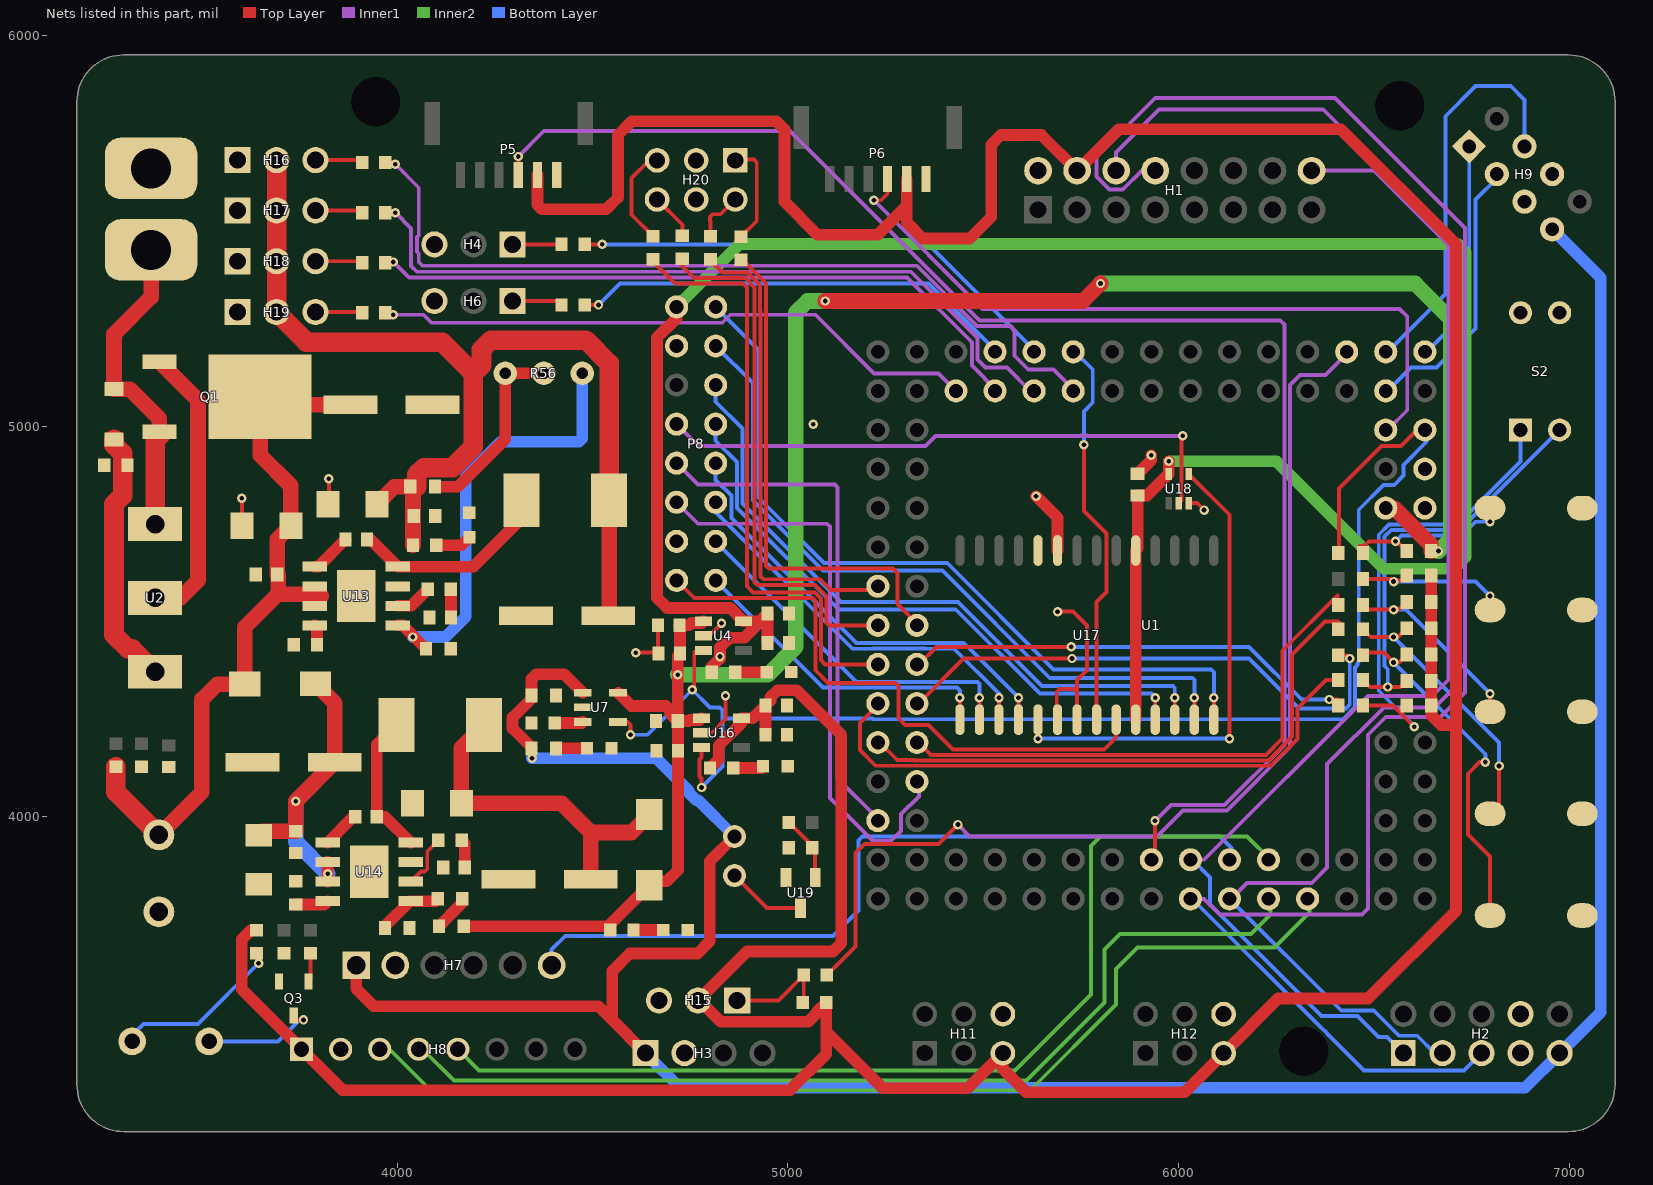
[diagram p0: the nets of this part, all layers, seen from the top]
# Altium PCB MISC49918.pcbdoc (part 2 of 2)
Units mil, origin at the board's own origin, x right, y up, seen from the top; angles counter-clockwise.
Board outline 3937.01 x 2755.91 mil, 4 copper layers (Top Layer, Inner1, Inner2, Bottom Layer), stack 62.447 mil thick; 130 components, 134 nets, 493 pads, 82 vias.

## Via types
v1: diameter 24.02, hole 12, Top Layer to Bottom Layer, 82 vias

## Nets (pads, with @x,y where several pads share a name; then routed paths per layer and width w, separated by ;. In a path a pad name is that pad's centre, name@x,y a point inside that pad or via, vN(x,y) a via of type N, cw(c..) or ccw(c..) an arc to the next point about the centre after c; other vN are vias at no path point) (continued)
7.3: U1.25 U17.8 | length 1003.8
  Top Layer w10: v1(5757.5,4952.5) 5757.5,4782.5 5815,4725 5815,4575 5790,4550 U17.8@5790,4248.46
  Bottom Layer w10: U1.25@5734.65,5190 5780,5144.65 5780,5060 5757.5,5037.5 v1(5757.5,4952.5)
7.4: R83.1 U1.45 | length 1218.1
  Top Layer w10: R83.1@4805,5420.34 4832.48,5392.86 4896.78,5392.86 4928.84,5360.81 4928.84,5294.02 4930,5292.86 4930,4615 4937.07,4607.93 5082.07,4607.93 5110,4580 5224.65,4580 U1.45@5234.65,4590
7.5: R61.2 U1.47 | length 1378.5
  Top Layer w10: R61.2@4730,5420.34 4730,5408.85 4760,5378.85 4890.98,5378.85 4914.82,5355 4914.82,4600 4921.89,4592.93 5069.64,4592.93 5098.03,4564.54 5098.03,4497.07 5105.1,4490 U1.47@5234.65,4490
7.6: R63.1 U1.48 | length 1312
  Top Layer w10: R63.1@4880,5425.34 4884.12,5425.34 4944.02,5365.45 4944.02,4642.07 4951.09,4635 5268.44,4635 5280,4623.44 5280,4544.65 U1.48@5334.65,4490
7.7: R62.2 U1.49 | length 1546.3
  Top Layer w10: R62.2@4655.62,5420.34 4711.13,5364.83 4885.17,5364.83 4895,5355 4895,4590 4910.98,4574.02 5068.73,4574.02 5084.02,4558.73 5084.02,4400.98 5095,4390 U1.49@5234.65,4390
8.0: P5.3 U1.74 | length 3829.6
  Top Layer w10: P5.3@4309.61,5642.32 4310,5642.72 v1(4310,5690) ; U1.74@5934.65,3890 5939.46,3894.81 v1(5939.46,3989.46)
  Inner1 w10: v1(4310,5690) 4375,5755 5005,5755 5490,5270 6260,5270 6270.51,5259.49 6270.51,4183.16 6117.35,4030 5980,4030 v1(5939.46,3989.46)
8.1: H1.8 H2.5 U1.75 | length 4720.8
  Inner1 w10: H1.8@5940,5653.7 5905.64,5653.7 5856.94,5605 5823.06,5605 5789.15,5638.91 5789.15,5689.15 5940,5840 6400,5840 6733.06,5506.94 6733.06,4318.06 6670,4255 6530,4255 6485,4210 6485,3765 6469.49,3749.49 6105.51,3749.49 6065,3790 U1.75@6034.65,3790
  Bottom Layer w10: U1.75@6034.65,3790 6363.9,3460.74 cw(c6320.01,3400.01) 6380.74,3443.9 6474.09,3350.55 6730.55,3350.55 H2.5@6775,3395
8.2: H1.16 H2.1 U1.76 | length 3174.3
  Inner1 w10: U1.76@6034.65,3890 6065,3890 6484.02,4309.02 6649.02,4309.02 6690,4350 6690,5463.7 6500,5653.7 H1.16@6340,5653.7
  Bottom Layer w10: U1.76@6035,3890 6080,3845 6080,3775 6365,3490 6457.53,3490 6511,3436.54 6533.46,3436.54 H2.1@6575,3395
8.3: H1.6 H2.3 U1.77 | length 3902.6
  Inner1 w10: H1.6@5840,5653.7 5840,5700 5950,5810 6370,5810 6710,5470 6710,4335 6655,4280 6525,4280 6380,4135 6380,3870 6340.51,3830.51 6175.16,3830.51 U1.77@6134.65,3790
  Bottom Layer w10: U1.77@6130,3790 6415.98,3504.02 6499.2,3504.02 6563.76,3439.45 6610.55,3439.45 6655,3395 H2.3@6675,3395
8.4: H7.6 U1.78 | length 2047.4
  Bottom Layer w10: H7.6@4395,3620 4395,3660 4430,3695 5115.18,3695 5180,3759.82 5180,3939.49 5190,3949.49 6105.51,3949.49 6135,3920 U1.78@6135,3890
8.5: H8.4 U1.79 | length 2508.3
  Inner2 w10: H8.4@4055.01,3405.02 4064.98,3405.02 4145,3325 5610,3325 5810,3525 5810,3660 5850,3700 6185,3700 6235,3750 U1.79@6235,3790
8.6: H8.5 U1.80 | length 2598.3
  Inner2 w10: H8.5@4155.01,3405.02 4209.47,3350.55 5580.55,3350.55 5775.51,3545.51 5775.51,3925.51 5800,3950 6175,3950 U1.80@6235,3890
8.7: H8.3 U1.81 | length 2699.7
  Inner2 w10: H8.3@3955.01,3405.02 3979.98,3405.02 4085,3300 5620,3300 5840,3520 5840,3610 5895,3665 6245,3665 6335,3755 U1.81@6335,3790
9.0: P6.3 U1.6 | length 1878.5
  Top Layer w10: v1(5220,5577.93) 5237.93,5577.93 5254.61,5594.61 P6.3@5254.61,5632.34
  Inner1 w10: v1(5220,5577.93) 5497.93,5300 6565,5300 6585,5280 6585,5040.35 U1.6@6534.65,4990
9.2: H9.3 U1.8 | length 709.1
  Bottom Layer w10: U1.8@6534.65,5090 6594.13,5149.49 6659.49,5149.49 6760,5250 6760,5580 6814.29,5634.29 H9.3@6814.29,5645
9.3: H9.1 U1.9 | length 570.8
  Bottom Layer w10: U1.9@6634.65,5190 6743.58,5298.93 H9.1@6743.58,5715.71
9.4: H9.4 U1.10 | length 1032.1
  Bottom Layer w10: U1.10@6534.65,5190 6682.93,5338.28 6682.93,5792.93 6760,5870 6850,5870 6885,5835 H9.4@6885,5715.71
9.6: R77.1 U1.11 | length 2704.4
  Top Layer w10: R77.1@5099.66,3595 5172.93,3668.27 5172.93,3907.93 5195.51,3930.51 5385.51,3930.51 v1(5435,3980)
  Inner1 w10: v1(5435,3980) 5465,3950 5945,3950 6010.98,4015.98 6123.16,4015.98 6285,4177.83 6285,5105 6310.51,5130.51 6375.51,5130.51 U1.11@6435,5190
$1N71: Q1.2 U2.2 | length 722.3
  Top Layer w40: U2.2@3380,4560 3445,4560 3490,4605 3490,5065.83 Q1.2@3396.06,5159.76
$1N72: D1.2 R1.2 U2.3 | length 662.7
  Top Layer w50: D1.2@3275,4965.63 3275,4952.04 3297.2,4929.84 3297.2,4822.2 3275,4800 3275,4465.36 3310.36,4430 3321.02,4430 U2.3@3380,4371.02
$1N74: D1.1 P1.1 Q1.3 U2.1 | length 814.6
  Top Layer w40: P1.1@3370,5450.67 3370,5330 3275,5235 D1.1@3275,5094.37 3315.63,5094.37 3391.06,5018.94 Q1.3@3391.06,4985.24
  Top Layer w50: U2.1@3380,4748.98 3380,4964.17 Q1.3@3396.06,4980.24
$1N79: LED8.2 R21.2 | length 79.1
  Top Layer w30: R21.2@4406.5,4175 4406.7,4175.2 LED8.2@4485.5,4175.2
$1N81: R22.2 U7.3 | length 72.7
  Top Layer w30: R22.2@4402.95,4240 4471.98,4240 U7.3@4474.58,4242.6
$1N85: C38.1 L3.1 U13.8 | length 522.3
  Top Layer w30: C38.1@3922.56,4710 3931.3,4710 U13.8@4001.3,4640 4195,4640 4317.8,4762.8 L3.1@4317.8,4810
$1N87: R47.1 R56.2 R56.3 | length 497.3
  Top Layer w30: R47.1@4096.5,4845 4155,4845 4276.57,4966.57 R56.3@4276.57,5135 R56.2@4375,5135
$1N88: R45.1 U13.6 | length 94.3
  Top Layer w30: U13.6@4001.3,4540 4035.27,4540 R45.1@4077.91,4582.63
$1N90: R49.2 R56.1 U13.5 | length 1117.1
  Top Layer w30: U13.5@4001.3,4490 4013.5,4490 R49.2@4073.5,4430
  Bottom Layer w30: v1(4040,4460) 4122.57,4460 4175,4512.43 4175,4870 4265,4960 4465,4960 4473.43,4968.43 R56.1@4473.43,5135
$1N91: LED4.2 R46.2 | length 93.6
  Top Layer w30: R46.2@4099.66,4695 4164.3,4695 LED4.2@4184.8,4715.5
$1N92: C39.2 R45.2 | length 72.8
  Top Layer w30: R45.2@4137.23,4582.63 4137.56,4582.3 C39.2@4137.56,4510
$1N93: C38.2 U13.1 | length 107.7
  Top Layer w30: U13.1@3788.7,4640 3797.44,4640 C38.2@3867.44,4710
$1N95: R44.2 U13.4 | length 52.5
  Top Layer w30: U13.4@3788.7,4490 3794.66,4484.04 R44.2@3794.66,4440
$1N99: LED9.2 R18.2 | length 80.9
  Top Layer w30: R18.2@4864.66,4370 4945.3,4370 LED9.2@4945.5,4370.2
$1N104: LED11.2 R58.2 | length 78.3
  Top Layer w30: R58.2@4859.66,4125 4931.84,4125 LED11.2@4936.15,4129.3
$1N111: C63.1 L4.1 U14.8 | length 369.8
  Top Layer w30: L4.1@3997.8,4235 3947.56,4184.77 C63.1@3947.56,4000 3968.41,4000 U14.8@4034.3,3934.1
$1N112: C65.1 C67.2 D7.A L4.2 | length 875.1
  Top Layer w40: L4.2@4222.2,4235 4164.04,4176.83 C67.2@4164.04,4034.81 4420.19,4034.81 4495.11,3959.89 ; C65.1@4495.11,3840 4495.11,3959.89 ; D7.A@4645,4005.55 4599.33,3959.89 4495.11,3959.89
$1N114: R53.1 R54.2 | length 94.8
  Top Layer w30: R53.1@4107,3719.81 4133.26,3746.07 4133.26,3746.21 4166.5,3779.45 R54.2@4166.5,3790
$1N115: R51.1 U14.6 | length 141.1
  Top Layer w10: U14.6@4034.3,3834.1 4060.53,3860.33 4070.35,3860.33 4076.79,3866.76 4076.79,3911.45 R51.1@4105.34,3940
$1N117: R54.1 R55.2 U14.5 | length 164
  Top Layer w30: R55.2@3968.5,3720 4032.61,3784.1 U14.5@4034.3,3784.1 4097.61,3784.1 R54.1@4103.5,3790
$1N118: LED5.2 R52.2 | length 75.9
  Top Layer w30: R52.2@4604.66,3710 4680.3,3710 LED5.2@4680.5,3710.2
$1N119: C64.2 R51.2 | length 73.3
  Top Layer w30: R51.2@4164.66,3940 4172.56,3932.1 C64.2@4172.56,3870
$1N120: C63.2 U14.1 | length 98
  Top Layer w30: U14.1@3821.71,3934.1 3887.6,4000 C63.2@3892.44,4000
$1N121: C61.1 C62.2 C66.2 D6.2 U14.2 U14.3 | length 808.5
  Top Layer w30: U14.3@3821.71,3834.1 v1(3821.71,3854.19) U14.2@3821.71,3884.1
  Top Layer w40: C66.2@3645,3952.7 3654.86,3962.56 C62.2@3740,3962.56 3740,4039.89 C61.1@3840.11,4140 3840.11,4290.96 D6.2@3790.7,4340.37
  Bottom Layer w40: v1(3740,4040) 3740,3935.9 v1(3821.71,3854.19)
$1N123: R50.2 U14.4 | length 85.3
  Top Layer w30: R50.2@3740,3775.34 3812.94,3775.34 U14.4@3821.71,3784.1
$2N19: H6.1 R60.1 | length 129.5
  Top Layer w10: H6.1@4295.01,5319.98 4410.36,5319.98 R60.1@4420.34,5310
$2N22: H4.1 R59.1 | length 125.3
  Top Layer w10: H4.1@4295.01,5465 R59.1@4420.34,5465
$2N45: H18.3 R81.1 | length 120.6
  Top Layer w10: H18.3@3790.94,5421.81 3906.09,5421.81 R81.1@3909.91,5417.98
$2N46: H19.3 R82.1 | length 119.8
  Top Layer w10: H19.3@3790.94,5291.77 3907.79,5291.77 R82.1@3909.91,5289.65
$2N51: H16.3 R79.1 | length 121.4
  Top Layer w10: H16.3@3790.94,5680.58 3903.99,5680.58 R79.1@3909.91,5674.65
$2N52: H17.3 R80.1 | length 121.3
  Top Layer w10: H17.3@3790.94,5551.84 3904.39,5551.84 R80.1@3909.91,5546.32
$2N64: H15.1 R77.2 R78.1 | length 268.6
  Top Layer w10: H15.1@4870,3530 4975.34,3530 R77.2@5040.34,3595 5040.34,3526.55 R78.1@5038.3,3524.5
$2N71: H20.5 R62.1 | length 255
  Top Layer w10: R62.1@4654.55,5486.18 4600,5540.73 4600,5635 4644.91,5679.91 H20.5@4664.99,5679.91
$2N72: H20.6 R61.1 | length 119.5
  Top Layer w10: H20.6@4664.99,5579.91 4729.61,5515.28 R61.1@4729.61,5487.15
$2N73: H20.1 R63.2 | length 265.7
  Top Layer w10: H20.1@4864.99,5679.91 4867.15,5682.07 4912.93,5682.07 4920,5675 4920,5524.66 R63.2@4880,5484.66
$2N74: H20.2 R83.2 | length 133
  Top Layer w10: R83.2@4801.44,5486.18 4801.44,5523.56 4800,5525 4800,5535 4807.07,5542.07 4827.15,5542.07 H20.2@4864.99,5579.91
$2N77: R84.2 R85.2 U19.1 | length 168.4
  Top Layer w10: R84.2@5002.45,3985.39 5061.77,3926.07 R85.2@5061.77,3920.39 5069.51,3912.65 U19.1@5069.51,3844.75
$2N78: P7.2 U19.3 | length 203.5
  Top Layer w10: P7.2@4863.2,3849.46 4946.65,3766.01 U19.3@5032.11,3766.01
$2N123: P8.2 U17.14 | length 2005.6
  Top Layer w10: U17.14@6090,4248.46 v1(6090,4305)
  Bottom Layer w10: P8.2@4815,5305 4925,5195 4925,4816.41 5091.92,4649.49 5407.58,4649.49 5680,4377.07 6082.93,4377.07 6090,4370 v1(6090,4305)
$2N124: P8.4 U17.13 | length 1856.8
  Top Layer w10: U17.13@6040,4248.46 v1(6040,4305)
  Bottom Layer w10: P8.4@4815,5205 4910,5110 4910,4810 5090,4630 5217.35,4630 5217.86,4630.51 5351.43,4630.51 5351.94,4630 5395,4630 5670,4355 6035,4355 6040,4350 v1(6040,4305)
$2N125: P8.6 U17.12 | length 1715.2
  Top Layer w10: U17.12@5990,4248.46 v1(5990,4305)
  Bottom Layer w10: P8.6@4815,5105 4815,5062.29 4883.54,4993.75 4883.54,4801.46 5135.51,4549.49 5435.51,4549.49 5650,4335 5985,4335 5990,4330 v1(5990,4305)
$2N126: P8.8 U17.11 | length 1565.6
  Top Layer w10: U17.11@5940,4248.46 v1(5940,4305)
  Bottom Layer w10: P8.8@4815,5005 4815,4962.29 4869.53,4907.76 4869.53,4790.47 5130,4530 5217.35,4530 5217.86,4530.51 5429.49,4530.51 5645,4315 5930,4315 v1(5940,4305)
$2N127: P8.10 U17.4 | length 1138.6
  Top Layer w10: U17.4@5590,4248.46 v1(5590,4305)
  Bottom Layer w10: P8.10@4815,4905 4815,4862.29 4855.51,4821.78 4855.51,4764.49 5175,4445 5449.7,4445 5460,4434.7 5460.3,4434.7 v1(5590,4305)
$2N128: P8.12 U17.3 | length 1009.6
  Top Layer w10: U17.3@5540,4248.46 v1(5540,4305)
  Bottom Layer w10: P8.12@4815,4805 4815,4780 5165,4430 5217.35,4430 5217.86,4430.51 5351.43,4430.51 5351.94,4430 5425,4430 5540,4315 v1(5540,4305)
$2N129: P8.14 U17.2 | length 917.7
  Top Layer w10: U17.2@5490,4248.46 v1(5490,4305)
  Bottom Layer w10: P8.14@4815,4705 5175,4345 5485,4345 5490,4340 v1(5490,4305)
$2N130: P8.16 U17.1 | length 816.6
  Top Layer w10: U17.1@5440,4248.46 v1(5440,4305)
  Bottom Layer w10: P8.16@4815,4605 5089.49,4330.51 5432.93,4330.51 5440,4323.44 v1(5440,4305)
$2N133: R95.2 R98.2 S2.1 | length 1203.7
  Top Layer w10: R98.2@6471.5,4285 6548.2,4285 v1(6602.69,4230.51)
  Bottom Layer w10: v1(6602.69,4230.51) 6602.69,4231.8 6512.01,4322.48 6512.01,4721.83 6538.21,4748.03 6713.22,4748.03 6874.99,4909.8 S2.1@6874.99,4989.98
$2N134: R96.2 R97.2 S2.2 | length 1075.2
  Top Layer w10: R97.2@6471.5,4350 6489.49,4332.01 v1(6535,4332.01) 6568.01,4332.01 R96.2@6583.5,4347.5
  Bottom Layer w10: v1(6535,4332.01) 6535,4377.48 6527.01,4385.48 6527.01,4717.01 6544.02,4734.02 6719.02,4734.02 S2.2@6974.99,4989.98
$2N139: R74.2 R76.2 S7.2 | length 452.9
  Top Layer w10: R76.2@6471.5,4675 6471.5,4685.86 6464.43,4692.93 6474.43,4692.93 6486.5,4705 v1(6555,4705) 6558.5,4705 R74.2@6583.5,4680 ; v1(6796.89,4755) S7.2@6796.89,4790
  Bottom Layer w10: v1(6555,4705) 6570,4720 6724.83,4720 6759.83,4755 v1(6796.89,4755)
$2N143: R86.2 R93.2 S6.2 | length 409
  Top Layer w10: R86.2@6471.5,4608.33 v1@6543.67,4608.33 ; v1@6550,4604.51 6570.51,4604.51 R93.2@6583.5,4617.5 ; S6.2@6796.89,4529.33 v1(6796.89,4565)
  Bottom Layer w10: v1(6550,4602.01) 6759.88,4602.01 v1(6796.89,4565)
$2N144: R87.2 R92.2 S5.2 | length 507.4
  Top Layer w10: R87.2@6471.5,4541.67 6483.16,4530 v1(6550,4530) 6563.5,4530 R92.2@6583.5,4550 ; S5.2@6796.89,4268.65 v1(6796.89,4315)
  Bottom Layer w10: v1(6550,4530) 6581.89,4530 v1(6796.89,4315)
$2N145: R88.2 R91.2 S4.2 | length 703
  Top Layer w10: R88.2@6471.5,4480 6491.5,4460 v1(6550,4460) 6561,4460 R91.2@6583.5,4482.5 ; S4.2@6796.89,4007.98 6820,4031.09 v1(6820,4130)
  Bottom Layer w10: v1(6550,4460) 6820,4190 v1(6820,4130)
$2N146: R89.2 R94.2 S3.2 | length 929.4
  Top Layer w10: R89.2@6471.5,4413.33 6478.16,4420 6525,4420 v1(6550,4395) 6563.5,4395 R94.2@6583.5,4415 ; v1(6785,4140) 6770,4140 6740,4110 6740,3955 6796.89,3898.11 S3.2@6796.89,3747.31
  Bottom Layer w10: v1(6550,4395) 6785,4160 v1(6785,4140)
$2N153: B1.1 R64.2 | length 443.7
  Top Layer w10: R64.2@3639.79,3650.55 3645,3645.35 v1(3645,3625)
  Bottom Layer w10: B1.1@3321.56,3424.99 3321.56,3441.56 3350,3470 3490,3470 v1(3645,3625)
$2N155: B1.2 Q3.3 | length 294.2
  Top Layer w10: Q3.3@3735,3491.64 3746.64,3480 v1(3760,3480)
  Bottom Layer w10: B1.2@3518.4,3424.99 3694.99,3424.99 3750,3480 v1(3760,3480)
$2N156: Q3.1 R33.2 | length 74.5
  Top Layer w10: Q3.1@3772.4,3578.36 3778.02,3583.98 R33.2@3778.02,3650.55
A.0: R79.2 U1.26 | length 2160.9
  Top Layer w10: R79.2@3969.23,5674.65 3990.35,5674.65 v1(3995,5670)
  Inner1 w10: v1(3995,5670) 4055,5610 4055,5487.85 4050.56,5483.41 4050.56,5446.59 4055,5442.15 4055,5420.23 4065,5410.23 5329.95,5410.23 5484.19,5255.98 5569.02,5255.98 5580,5245 5580,5180 5615,5145 5680,5145 U1.26@5735,5090
A.1: R59.2 U1.27 | length 1268.9
  Top Layer w10: R59.2@4479.66,5465 v1(4525,5465)
  Bottom Layer w10: v1(4525,5465) 5359.65,5465 U1.27@5634.65,5190
A.2: R80.2 U1.28 | length 1943.4
  Top Layer w10: R80.2@3969.23,5546.32 v1(3995,5546.32)
  Inner1 w10: v1(3995,5546.32) 4035.23,5506.09 4035.23,5409.77 4050,5395 5315,5395 5485,5225 5485,5170 5505.51,5149.49 5560.51,5149.49 5620,5090 U1.28@5635,5090
A.3: R60.2 U1.29 | length 1150.3
  Top Layer w10: R60.2@4479.66,5310 v1(4515,5310)
  Bottom Layer w10: v1(4515,5310) 4570,5365 5359.65,5365 U1.29@5534.65,5190
A.4: R81.2 U1.30 | length 1738.4
  Top Layer w10: R81.2@3969.23,5417.98 3987.98,5417.98 v1(3990,5420)
  Inner1 w10: v1(3990,5420) 4030,5380 5305,5380 5470.51,5214.49 5470.51,5154.49 U1.30@5535,5090
A.6: R82.2 U1.32 | length 1565.5
  Top Layer w10: R82.2@3969.23,5289.65 3985.35,5289.65 v1(3990,5285)
  Inner1 w10: v1(3990,5285) 4067.13,5285 4087.64,5264.49 4831.78,5264.49 4852.29,5285 5070,5285 5220,5135 5385,5135 U1.32@5430,5090 U1.32@5435,5090
B.0: R98.1 U1.50 | length 1148.4
  Top Layer w10: U1.50@5334.65,4390 5379.65,4435 v1(5725,4435) ; v1(6385,4300) R98.1@6408.5,4300
  Bottom Layer w10: v1(5725,4435) 6180,4435 6315,4300 v1(6385,4300)
B.1: R97.1 U1.51 | length 1517.1
  Top Layer w10: U1.51@5234.65,4290 5184.49,4239.84 5184.49,4170.51 5224.49,4130.51 6235.33,4130.51 6304.02,4199.19 6304.02,4276.61 6377.41,4350 R97.1@6408.5,4350
B.2: R89.1 U1.52 | length 1358.6
  Top Layer w10: U1.52@5334.65,4290 5449.65,4405 v1(5727.01,4405) ; R89.1@6408.5,4413.33 6429.42,4413.33 v1(6437.76,4405)
  Bottom Layer w10: v1(5727.01,4405) 6180,4405 6307.99,4277.01 6427.76,4277.01 6437.76,4287.01 v1(6437.76,4405)
B.3: R88.1 U1.53 | length 1487.8
  Top Layer w10: U1.53@5234.65,4190 5279.65,4145 5322.35,4145 5322.83,4144.53 6229.53,4144.53 6290,4205 6290,4415 6375,4500 6408.5,4500 6414.36,4494.14 6414.36,4485.86 R88.1@6408.5,4480
B.4: R87.1 U1.54 | length 1411.7
  Top Layer w10: U1.54@5334.65,4190 5366.1,4158.54 6223.54,4158.54 6265,4200 6265,4425 6406.67,4566.67 6406.67,4543.5 R87.1@6408.5,4541.67
B.6: P8.11 U1.56 | length 1496.8
  Inner1 w10: P8.11@4715,4805 4770,4750 5100,4750 5107.07,4742.93 5107.07,4047.93 5217.51,3937.49 5263,3937.49 5289.49,3963.98 5289.49,4006.78 5335,4052.29 U1.56@5335,4090
B.7: P8.9 U1.57 | length 1335.4
  Inner1 w10: P8.9@4715,4905 4770,4850 5120,4850 5127.07,4842.93 5127.07,4097.93 U1.57@5235,3990
GND: C18.1 C29.1 C35.2 C37.1 C39.1 C43.1 C53.2 C59.1 C60.1 C61.2 C62.1 C64.1 C65.2 C66.1 C67.1 C68.1 C71.1 C72.1 C73.1 C74.1 C75.1 C76.1 C77.1 C78.1 H1.2 H2.7 H2.8 H3.2 H4.3 H6.3 H7.2 H8.2 H9.5 H9.6 H11.6 H12.6 H15.3 H16.1 H17.1 H18.1 H19.1 H20.3 H20.4 LED4.1 LED5.1 LED8.1 LED9.1 LED11.1 P1.2 P4.1 P5.1 P6.1 P8.3 P8.13 Q3.2 R1.1 R22.1 R34.2 R44.1 R49.1 R50.1 R55.1 R85.1 R99.1 S2.3 S2.4 S3.1 S4.1 S5.1 S6.1 S7.1 U1.1 U1.3 U4.2 U7.2 U13.7 U13.9 U14.7 U14.9 U16.2 U17.6 U17.7 U17.23 U17.24 U18.3 U19.2 | length 1203.7
  Top Layer w10: C59.1@3602.19,4744.58 v1(3602.19,4815) ; C60.1@3822.3,4800 3825,4802.7 v1(3825,4865) ; v1(4610,4420) 4666.5,4420 C71.1@4667.44,4419.06 ; C18.1@4667.44,4490 C71.1@4667.44,4419.06 ; C71.1@4668.38,4418.12 C71.1@4667.44,4419.06 ; U16.2@4778.82,4215 4805,4215 4840,4250 v1(4840,4310) ; U4.2@4783.42,4463.12 4798.12,4463.12 v1(4830,4495) ; U17.6@5690,4248.46 5687.93,4250.54 5687.93,4320 5695,4327.07 5732.93,4327.07 5740,4320 ; v1(5690,4525) 5730,4525 5765,4490 5765,4375 5740,4350 5740,4320 ; U17.7@5740,4248.46 5740,4320 ; U18.3@6025.59,4802.6 6047.4,4802.6 v1(6065,4785)
  Top Layer w30: v1(5635,4820) 5690,4765 U17.23@5690,4681.54 ; C77.1@5895,4877.56 5930,4912.56 v1(5930,4925)
  other v1: 5065,5005
HREF: P8.7 U18.2 | length 1505.5
  Top Layer w10: U18.2@6000,4802.6 6006.73,4809.33 6006.73,4971.73 v1(6010,4975)
  Inner1 w10: P8.7@4715,5005 4770.51,4949.49 5351.78,4949.49 5377.29,4975 5747.48,4975 5747.98,4975.49 5767.02,4975.49 5767.52,4975 v1(6010,4975)
PCLK: P8.15 U17.9 | length 1514.9
  Top Layer w10: P8.15@4715,4605 4760,4560 5062.93,4560 5070,4552.93 5070,4375 5102.93,4342.07 5275.86,4342.07 5282.93,4335 5282.93,4252.07 5300,4235 5360,4235 5422.44,4172.56 5809.45,4172.56 5840,4203.11 U17.9@5840,4248.46
RST: R76.1 U1.5 U4.3 U7.4 U16.3 | length 3701.9
  Top Layer w10: U7.4@4565.42,4242.6 4590,4242.6 4597.07,4235.53 v1(4597.07,4210) ; v1(4755,4325) 4760,4330 4760,4420 4767.07,4427.07 4782.07,4427.07 U4.3@4783.42,4425.72 ; v1(4778.82,4075) 4778.82,4098.1 4773.48,4103.44 4773.48,4146.56 4778.82,4151.9 U16.3@4778.82,4177.6 ; R76.1@6408.5,4675 6410,4676.5 6410,4840 6519.49,4949.49 6569.49,4949.49 6610,4990 U1.5@6634.65,4990
  Bottom Layer w10: v1(4597.07,4210) 4640,4210 v1(4755,4325) 4800,4280 4825,4280 4832.07,4272.93 4832.07,4251.15 ; v1(4778.82,4075) 4832.07,4128.25 4832.07,4251.15 ; U1.5@6635,4990 6635,4960 6575.51,4900.51 6575.51,4873.22 6551.78,4849.49 6524.49,4849.49 6460.75,4785.75 6460.75,4395.48 6457.75,4392.47 6457.75,4388.11 6451.77,4382.13 6451.77,4281.2 6420.06,4249.49 5218.22,4249.49 5216.56,4251.15 4832.07,4251.15
VCC3V3: C74.2 C76.2 H1.4 H8.1 H11.5 H12.5 H15.2 P5.2 P6.2 R58.1 R64.1 R78.2 R91.1 R92.1 R93.1 R94.1 R95.1 R96.1 U16.5 | length 11389.9
  Top Layer w30: R64.1@3639.79,3709.87 3624.87,3709.87 3601.8,3686.8 3601.8,3558.22 H8.1@3755.01,3405.02 3860.02,3300 5005,3300 5097.62,3392.62 5097.62,3449.5 ; P5.2@4358.82,5642.32 4358.82,5566.18 4370,5555 4535,5555 4565,5585 4565,5745 4600,5780 4970,5780 4991.21,5758.79 4991.21,5573.79 5075,5490 5230,5490 5303.83,5563.83 ; R58.1@4800.34,4125 4822.8,4147.46 4822.8,4182.36 4881.18,4240.74 U16.5@4881.18,4252.4 4909.84,4252.4 C74.2@4942.44,4285 ; C76.2@4942.44,4210 C74.2@4942.44,4285 ; P6.2@5303.83,5632.34 5303.83,5563.83 ; R93.1@6646.5,4617.5 R92.1@6646.5,4550 R91.1@6646.5,4482.5 R94.1@6646.5,4415 R96.1@6646.5,4347.5 R95.1@6646.5,4285 6646.5,4259.58 6671.08,4235 6700,4235 6710,4225 ; C74.2@4942.44,4285 4955,4297.56 4955,4305.58 4973.12,4323.7 5022,4323.7 5136.21,4209.49 5136.21,3676.21 5115,3655 4895,3655 H15.2@4770,3530 4775.5,3524.5 4778.89,3524.5 4827.84,3475.55 5051.91,3475.55 5075.16,3498.8 5075.16,3502.04 R78.2@5097.62,3524.5 5097.62,3449.5 ; 5097.62,3449.5 5242.12,3305 5460,3305 H11.5@5550,3395 5550,3355 5610,3295 6015,3295 H12.5@6115,3395 6255,3535 6485,3535 6710,3760 6710,4225 ; 5303.83,5563.83 5303.83,5521.4 5345.23,5480 5465,5480 5520,5535 5520,5720 5545,5745 5648.7,5745 H1.4@5740,5653.7 5846.3,5760 6415,5760 6710,5465 6710,4225
VCC5V: C18.2 C71.2 C73.2 C75.2 D7.K R52.1 R53.2 R74.1 U1.2 U4.1 U7.5 U16.1 | length 5298.9
  Top Layer w10: R74.1@6646.5,4680 v1(6665,4680)
  Top Layer w30: R53.2@4169.99,3719.81 4535.53,3719.81 R52.1@4545.34,3710 4545.34,3724.79 D7.K@4645,3824.45 4655.55,3835 4690,3835 4718.5,3863.5 C75.2@4718.5,4169.1 4718.5,4244.06 C73.2@4717.56,4245 ; U7.5@4565.42,4317.4 4599.12,4283.7 4686.88,4283.7 4699.17,4271.41 4699.17,4263.39 C73.2@4717.56,4245 ; U16.1@4778.82,4252.4 4774.21,4247.8 4748.47,4247.8 4745.68,4245 C73.2@4717.56,4245 ; U4.1@4783.42,4500.52 4778.81,4495.92 4753.07,4495.92 4747.16,4490 C18.2@4722.56,4490 4723.5,4489.06 C71.2@4723.5,4418.12 4717.56,4412.18 v1(4717.56,4363.49) C73.2@4717.56,4245
  Top Layer w40: v1(5095,5320) 5755,5320 v1(5800,5365) ; U1.2@6530,4790 6551.49,4790 6646.5,4695 R74.1@6646.5,4680
  Inner2 w40: v1(4717.56,4363.49) 4948.49,4363.49 5020,4435 5020,5290 5050,5320 v1(5095,5320) ; v1(5800,5365) 6605,5365 6695.98,5274.02 6695.98,4710.98 v1(6665,4680)
VCC5V_EXT: C29.2 H2.9 H3.1 H7.1 H9.7 P7.1 R21.1 U7.1 | length 7188
  Top Layer w10: v1(4345,4150) R21.1@4345,4173.5
  Top Layer w30: H7.1@3895,3620 3895,3560 3940,3515 4515,3515 4550,3480 ; R21.1@4343.5,4175 4343.5,4177.57 4295,4226.07 4295,4253.93 4343.5,4302.43 C29.2@4343.5,4310 4343.5,4352.43 4356.08,4365 4426.98,4365 U7.1@4474.58,4317.4 ; H3.1@4635,3395 4550,3480 ; P7.1@4863.2,3949.46 4800,3886.26 4800,3681.21 4768.79,3650 4595,3650 4550,3605 4550,3480
  Bottom Layer w30: v1(4345,4150) 4662.66,4150 4745.83,4066.83 4745.83,4061.33 4765.15,4042.01 4770.65,4042.01 P7.1@4863.2,3949.46 ; H3.1@4635,3395 4723.69,3306.31 6886.31,3306.31 H2.9@6975,3395 7080,3500 7080,5379.29 H9.7@6955.71,5503.58
VCCBAT: C35.1 C37.2 C59.2 D6.1 P4.2 Q1.1 R100.2 U13.2 U13.3 | length 1907.8
  Top Layer w40: P4.2@3390,3953.43 3500,4063.43 3500,4300 3539.63,4339.63 D6.1@3609.3,4339.63 3609.3,4484.3 3695,4570 ; 3805,4565 3800,4570 3695,4570 ; C35.1@3879.89,5055 3668.94,5055 Q1.1@3648.94,5075 3648.94,4926.06 3727.59,4847.41 C59.2@3727.59,4744.58 3692.56,4709.55 C37.2@3692.56,4620 3695,4617.56 3695,4570
  Top Layer w50: R100.2@3280,4127.53 3280,4063.43 P4.2@3390,3953.43
VCCCAM: C43.2 C72.2 C77.2 P8.1 R18.1 U4.5 U17.10 U17.19 U18.5 | length 5827.5
  Top Layer w30: P8.1@4715,5305 4715,5276.43 4664.49,5225.92 4664.49,4560.51 4690.46,4534.54 4851.77,4534.54 U4.5@4885.78,4500.52 4915.32,4500.52 ; R18.1@4805.34,4370 4805.34,4384.5 4826.06,4405.22 v1(4826.06,4410) 4826.06,4434 4850.57,4458.51 4888.51,4458.51 4915.32,4485.32 4915.32,4500.52 ; C72.2@4947.44,4445 C43.2@4947.44,4520 4927.96,4500.52 4915.32,4500.52 ; U17.10@5890,4248.46 U17.19@5890,4681.54 ; C77.2@5895,4822.44 5919.45,4822.44 U18.5@5974.41,4877.4 5974.41,4909.41 v1(5974.93,4909.93)
  Top Layer w30.01: U17.19@5890,4681.54 5895,4686.54 C77.2@5895,4822.44
  Inner2 w30: P8.1@4715,5305 4876.21,5466.21 6713.79,5466.21 6735,5445 6735,4665 6705,4635 6525,4635 6250.07,4909.93 v1(5974.93,4909.93)
VCCSERVO: C53.1 C60.2 C68.2 H16.2 H17.2 H18.2 H19.2 L3.2 R46.1 R47.2 | length 2686.7
  Top Layer w40: C60.2@3947.7,4800 3992.7,4845 R47.2@4033.5,4845 4040.34,4838.16 R46.1@4040.34,4695 ; C53.1@4540.11,4515 4542.2,4517.09 L3.2@4542.2,4810
  Top Layer w50: H16.2@3690.94,5680.58 H17.2@3690.94,5551.84 H18.2@3690.94,5421.81 H19.2@3690.94,5291.77 3767.72,5215 4115,5215 4194.25,5135.75 4194.25,4946.5 4141.45,4893.7 4067.91,4893.7 4049.76,4875.55 4049.76,4845 R47.2@4033.5,4845 ; 4205,5145 4215.59,5155.59 4215.59,5195.59 4240,5220 4482.83,5220 4542.2,5160.63 L3.2@4542.2,4810
WE: U17.5 U18.4 | length 1259.1
  Top Layer w10: v1(5640,4200) U17.5@5640,4248.46 ; U18.4@6025.59,4877.4 6130,4772.99 v1(6130,4200)
  Bottom Layer w10: v1(5640,4200) v1(6130,4200)
pads on no net: H1.1 H1.3 H1.5 H1.7 H1.9 H1.11 H1.13 H1.15 H2.2 H4.2 H6.2 H8.7 H8.8 H9.2 H11.1 H11.2 H12.1 H12.2 P5.0 P5.5 P5.6 P6.0 P6.5 P6.6 SCREW1.1 SCREW2.1 SCREW3.1 U1.4 U1.7 U1.12 U1.14 U1.17 U1.18 U1.19 U1.31 U1.33 U1.55 U1.58 U1.59 U1.61 U1.62 U1.64 U1.65 U1.66 U1.67 U1.70 U1.83 U1.86 U1.87 U1.88 U4.4 U16.4
copper on no net:
  other v1: 4615,5180 3315,5845 3345,5845 3315,5875 3345,5875

## Polygon pours and split planes (outlines as drawn)
GND on Top Layer (solid, remove dead copper, pour order 0): 3000,6205 3000,3045 7435,3045 7435,6205
GND on Bottom Layer (solid, remove dead copper, pour order 2): 3030,6125 3030,3000 7285,3000 7285,6125

## Keep-outs
Board Outline Layer:
  the board outline again, w10

## Other copper
Top Layer:
  text "2026.4.10" at 5470,5845 h51.18

## Silkscreen, mask and mechanical layers (free items; w line width, h text height)
Top Silkscreen Layer:
  text "Wireless serial port" at 6840,5865 h70 r315
  text "Servo connector" at 3520,5790 h70
  text "Display connector" at 5845,5750 h70
  text "-" at 3315,5745 h120
  text "Motor signal connector" at 4530,5745 h70
  text "Encoder 3" at 4117.39,5530 h70
  text "Encoder 4" at 5097.39,5515 h70
  text "Brushless ESC connector" at 4320,5355 h50
  text "+" at 3305,5240 h120
  text "Camera connector" at 4940,4730 h70 r90
  text "Voltage measurement" at 3275,4250 h50
  text "+" at 3175,3890 h120
  text "-" at 3334.5,3710 h120
  text "Laser connector" at 4749.91,3690 h60
  text "-" at 3175,3680 h120
  text "Motor power connector" at 3205,3590 h50
  text "Magnet sensor module connector" at 4500,3585 h60
  text "Encoder 1" at 5290,3560 h70
  text "Encoder 2" at 5872.39,3560 h70
  text "Wireless SPI" at 6609.89,3525 h70
  text "ToF module connector" at 3940,3480 h60
  text "Attitude sensor connector" at 3879.92,3285 h50
  text "Serial port connector" at 4655,3260 h60
Top Solder Mask Layer:
  text "COMPANY_A" at 4585,5850 h39.37
  text "2026.4.10" at 5470,5845 h51.18
  text "PERSON_A" at 5060,5835 h59.06